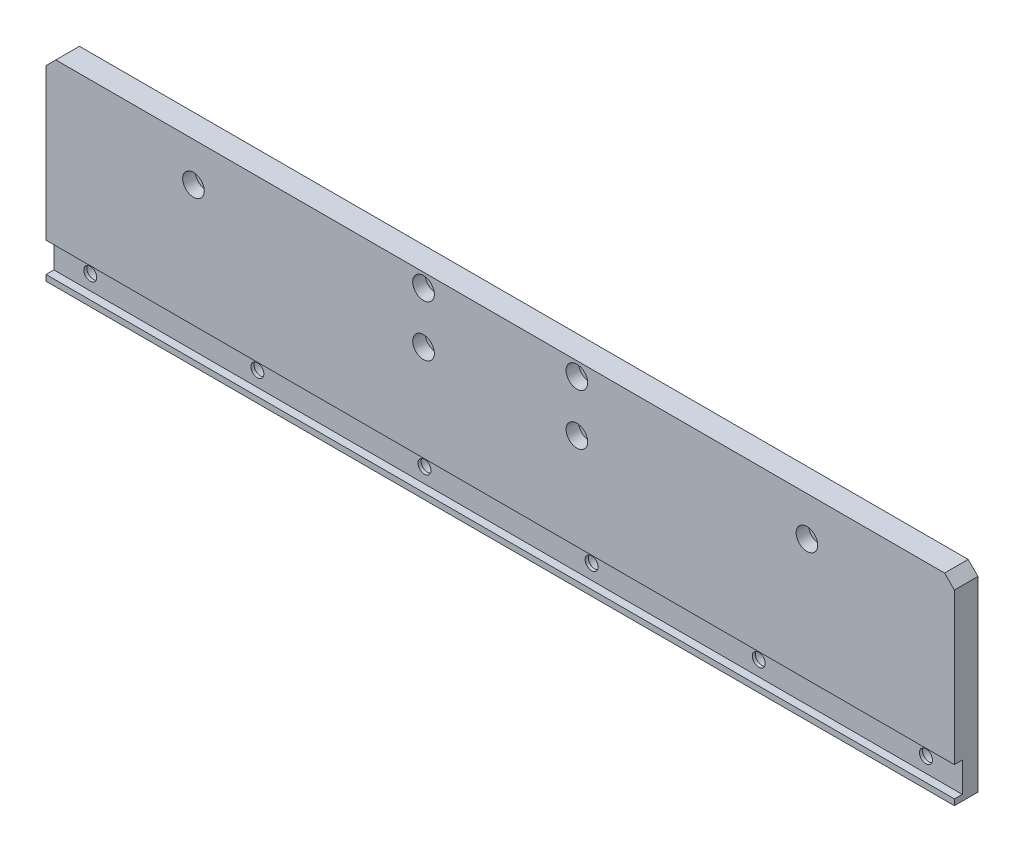
from build123d import *

# Parameters (mm, degrees)
SKETCH_1_W                   = 462
SKETCH_1_H                   = 100
EXTRUDE_1_DEPTH              = 12
SKETCH_2_W                   = 462
SKETCH_2_H                   = 15.1
CUT_EXTRUDE_1_DEPTH          = 4
HOLE_WIZARD_M6_1_D           = 6.6
HOLE_WIZARD_M6_1_CBORE_D     = 11
HOLE_WIZARD_M6_1_CBORE_DEPTH = 6.4
SKETCH_5_R                   = 10
CUT_EXTRUDE_2_DEPTH          = 2
HOLE_WIZARD_M6_2_D           = 6.6
HOLE_WIZARD_M6_2_CBORE_D     = 11
HOLE_WIZARD_M6_2_CBORE_DEPTH = 6.4
HOLE_WIZARD_M6_3_D           = 6.6
HOLE_WIZARD_M6_3_CBORE_D     = 11
HOLE_WIZARD_M6_3_CBORE_DEPTH = 6.4
CHAMFER_1_SIZE               = 5


with BuildPart() as part:
    # 草图1 → 凸台-拉伸1 (new body)
    with BuildSketch(Plane.XY):
        with Locations((231, 50)):
            Rectangle(SKETCH_1_W, SKETCH_1_H)
    extrude(amount=EXTRUDE_1_DEPTH)

    # 草图2 → 切除-拉伸1 (cut)
    with BuildSketch(Plane.XY.offset(12)):
        with Locations((231, 10.55)):
            Rectangle(SKETCH_2_W, SKETCH_2_H)
    extrude(amount=-CUT_EXTRUDE_1_DEPTH, mode=Mode.SUBTRACT)

    # M6 六角凹头螺钉的柱形沉头孔1 (through all)
    with Locations(Plane.XY.offset(12)):
        with Locations((192, 93), (270, 93), (192, 67), (270, 67)):
            CounterBoreHole(HOLE_WIZARD_M6_1_D / 2, HOLE_WIZARD_M6_1_CBORE_D / 2, HOLE_WIZARD_M6_1_CBORE_DEPTH)

    # 草图5 → 切除-拉伸2 (cut)
    with BuildSketch(Plane(origin=(0, 0, 0), x_dir=(-1, 0, 0), z_dir=(0, 0, -1))):
        with Locations((-387, 80)):
            Circle(SKETCH_5_R)
        with Locations((-75, 80)):
            Circle(SKETCH_5_R)
    extrude(amount=-CUT_EXTRUDE_2_DEPTH, mode=Mode.SUBTRACT)

    # M6 六角凹头螺钉的柱形沉头孔2 (through all)
    with Locations(Plane.XY.offset(12)):
        with Locations((75, 80), (387, 80)):
            CounterBoreHole(HOLE_WIZARD_M6_2_D / 2, HOLE_WIZARD_M6_2_CBORE_D / 2, HOLE_WIZARD_M6_2_CBORE_DEPTH)

    # M6 六角凹头螺钉的柱形沉头孔3 (through all)
    with Locations(Plane(origin=(0, 0, 0), x_dir=(-1, 0, 0), z_dir=(0, 0, -1))):
        with Locations((-443.5, 10.55), (-358.5, 10.55), (-273.5, 10.55), (-188.5, 10.55), (-103.5, 10.55), (-18.5, 10.55)):
            CounterBoreHole(HOLE_WIZARD_M6_3_D / 2, HOLE_WIZARD_M6_3_CBORE_D / 2, HOLE_WIZARD_M6_3_CBORE_DEPTH)

    # 倒角1
    chamfer_1_edges = [part.edges().sort_by_distance(p)[0] for p in [
        (0, 100, 6),
        (462, 100, 6),
    ]]
    chamfer(chamfer_1_edges, length=CHAMFER_1_SIZE)


solid = part.part
